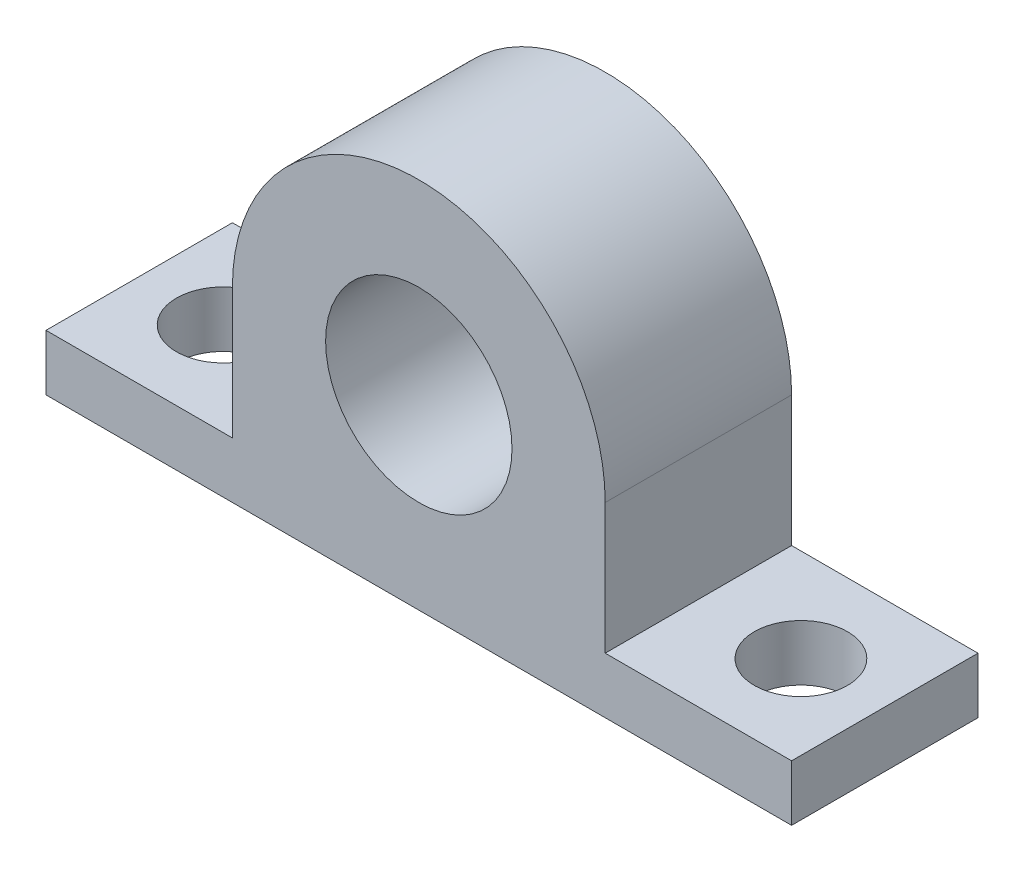
from build123d import *

# Parameters (mm, degrees)
SKETCH1_R           = 10
BOSS_EXTRUDE1_DEPTH = 10
SKETCH2_R           = 5
CUT_EXTRUDE1_DEPTH  = 10


with BuildPart() as part:
    # Sketch1 → Boss-Extrude1 (new, symmetric)
    with BuildSketch(Plane.XY):
        with BuildLine():
            Line((-40, -14), (-40, -20))
            Line((-40, -20), (40, -20))
            Line((40, -20), (40, -14))
            Line((40, -14), (20, -14))
            Line((20, -14), (20, 0))
            ThreePointArc((20, 0), (0, 20), (-20, 0))
            Line((-20, 0), (-20, -14))
            Line((-20, -14), (-40, -14))
        make_face()
        Circle(SKETCH1_R, mode=Mode.SUBTRACT)
    extrude(amount=BOSS_EXTRUDE1_DEPTH, both=True)

    # Sketch2 → Cut-Extrude1 (cut, symmetric)
    with BuildSketch(Plane(origin=(0, -14, 0), x_dir=(1, 0, 0), z_dir=(0, 1, 0))):
        with Locations(Location((31, 0, 0), (0, 0, 180))):
            Circle(SKETCH2_R)
        with Locations(Location((-31, 0, 0), (0, 0, 180))):
            Circle(SKETCH2_R)
    extrude(amount=CUT_EXTRUDE1_DEPTH, both=True, mode=Mode.SUBTRACT)


solid = part.part
